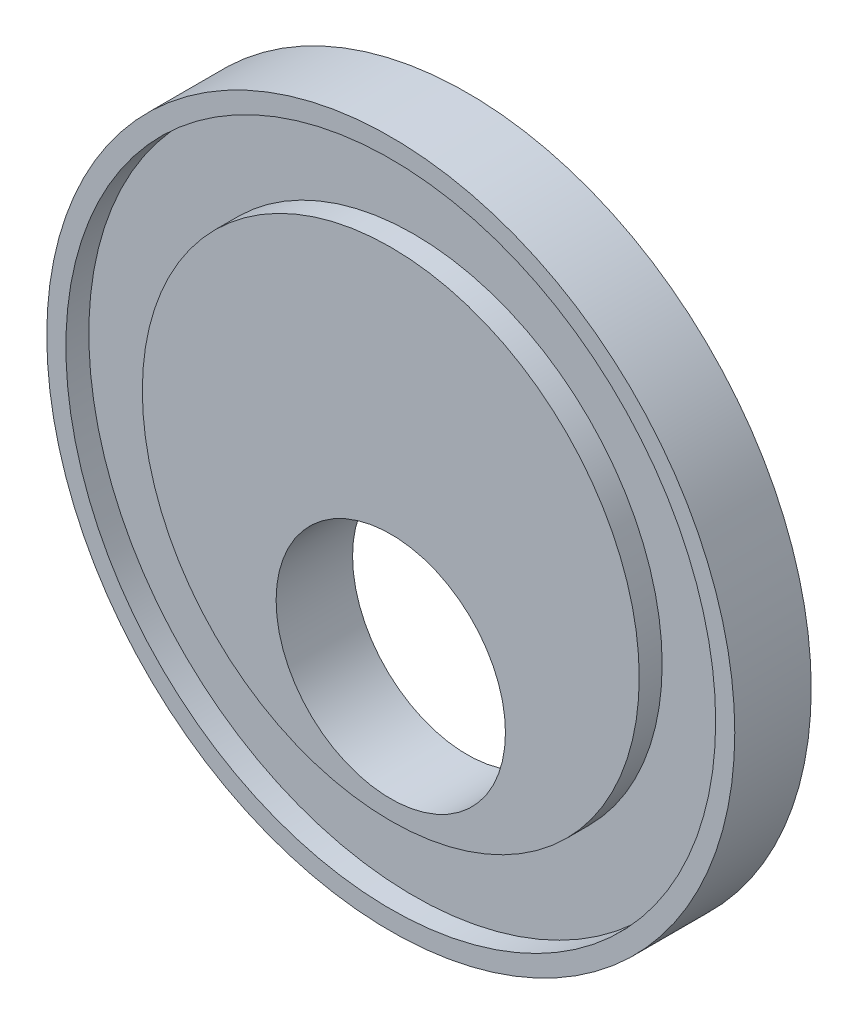
SolidWorks part; units mm, degrees
ref_plane "Front Plane" through (0, 0, 0) normal (0, 0, 1) x (1, 0, 0)
ref_plane "Top Plane" through (0, 0, 0) normal (0, 1, 0) x (1, 0, 0)
ref_plane "Right Plane" through (0, 0, 0) normal (1, 0, 0) x (0, 0, -1)
other "Configuration Table"
sketch "Sketch1" plane through (0, 0, 0) normal (0, 0, 1) x (1, 0, 0)
  circle A0 centre (0, 0) radius 30
  circle A1 centre (0, 30) radius 90
  dimension "D1" = 60
  dimension "D2" = 180
extrude "Boss-Extrude1" add sketch "Sketch1" along normal blind 20
sketch "Sketch2" plane through (0, 0, 20) normal (0, 0, 1) x (1, 0, 0)
  circle A0 centre (0, 30) radius 85
  circle A1 centre (0, 30) radius 65
  circle A2 centre (0, 30) radius 90 construction
  dimension "D1" = 5
  dimension "D2" = 20
extrude "Cut-Extrude1" cut sketch "Sketch2" against normal blind 6
sketch "Sketch3" plane through (0, 0, 0) normal (0, 0, -1) x (-1, 0, 0)
  circle A0 centre (0, 30) radius 85
  circle A1 centre (0, 30) radius 65
  circle A2 centre (0, 30) radius 90 construction
  dimension "D1" = 5
  dimension "D2" = 20
extrude "Cut-Extrude2" cut sketch "Sketch3" against normal blind 6
